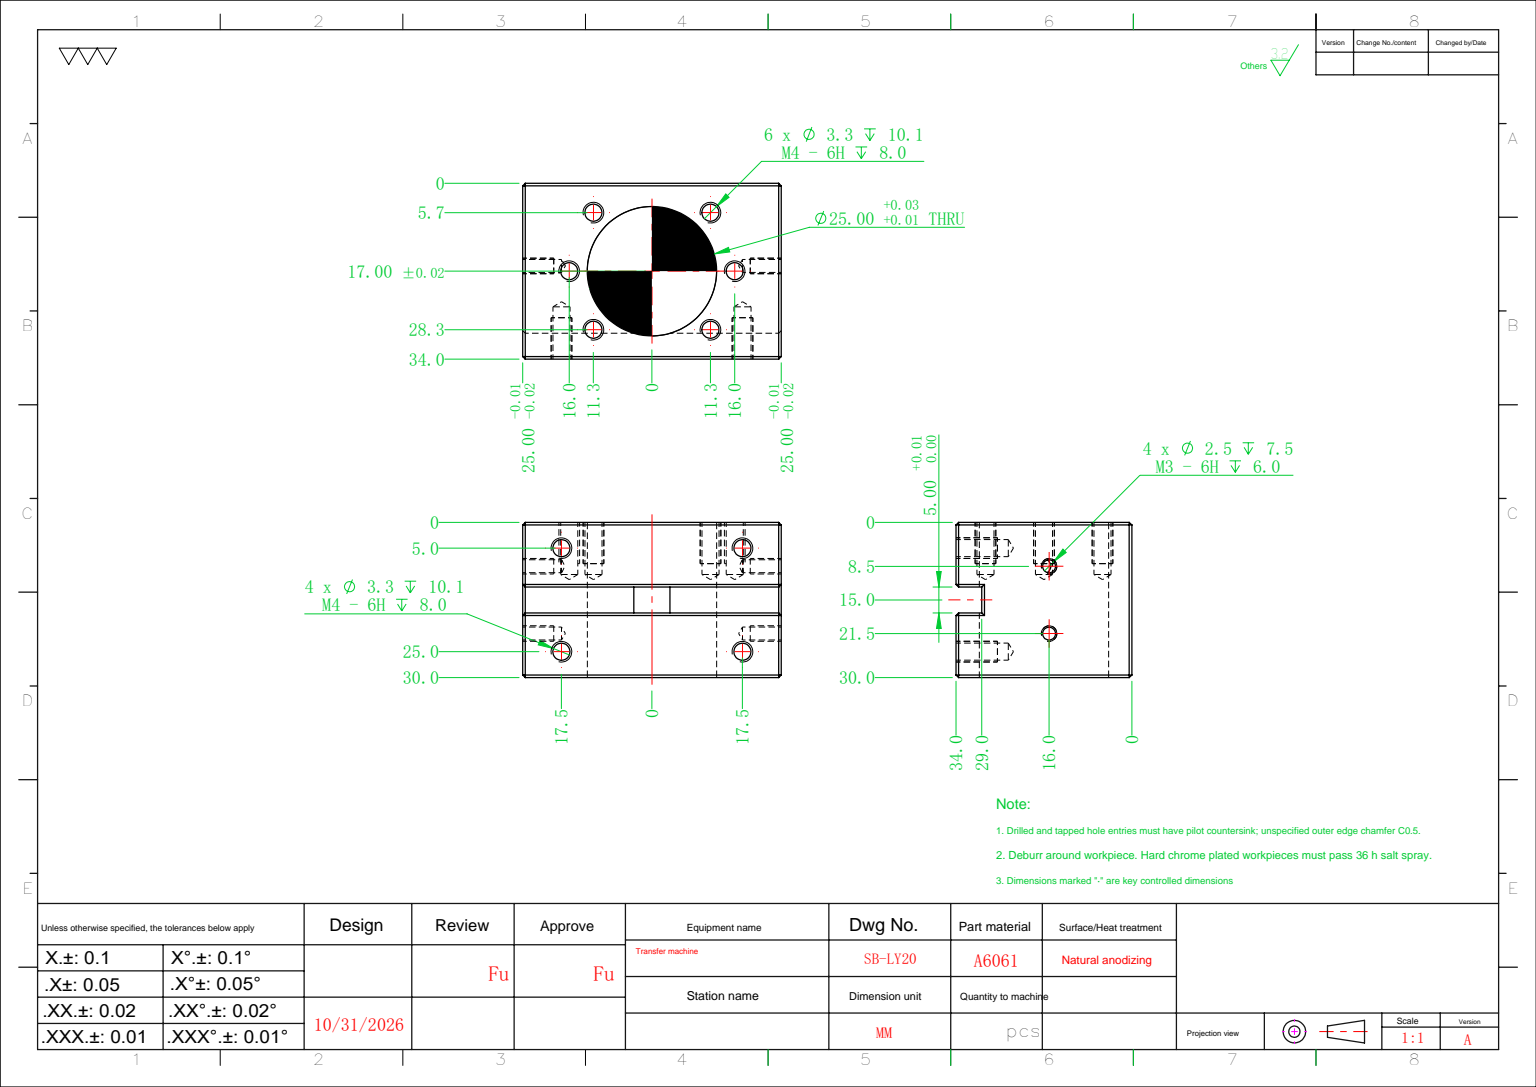
SolidWorks part; units mm, degrees
ref_plane "前视基准面" through (0, 0, 0) normal (0, 0, 1) x (1, 0, 0)
ref_plane "上视基准面" through (0, 0, 0) normal (0, 1, 0) x (1, 0, 0)
ref_plane "右视基准面" through (0, 0, 0) normal (1, 0, 0) x (0, 0, -1)
sketch "草图1" plane through (0, 0, 0) normal (0, 0, 1) x (1, 0, 0)
  line L1 (-25, -17) -> (25, -17)
  line L2 (-25, -17) -> (-25, 17)
  line L3 (-25, 17) -> (25, 17)
  line L4 (25, -17) -> (25, 17)
  line L5 (-25, -17) -> (25, 17) construction
  line L6 (-25, 17) -> (25, -17) construction
  point P0 (0, 0)
  dimension "D1" = 50
  dimension "D2" = 34
extrude "凸台-拉伸1" add sketch "草图1" along normal blind 30
hole_wizard "M4 螺纹孔1" positions "草图7" profile "草图8" tap size "M4" standard "ISO"
sketch "草图7" plane through (0, 0, 0) normal (0, 0, -1) x (-1, 0, 0)
  line L7 (0, 0) -> (0, 26.8833) construction
  line L9 (-16, 0) -> (16, 0) construction
  circle A0 centre (0, 0) radius 16 construction
  point P0 (-11.3137, -11.3137)
  point P3 (-16, 0)
  point P6 (-11.3137, 11.3137)
  point P9 (11.3137, 11.3137)
  point P12 (16, 0)
  point P15 (11.3137, -11.3137)
  dimension "D1" = 32
  dimension "D2" = 32
  dimension "D3" = 22.6274
sketch "草图8" plane through (11.3137, -11.3137, 0) normal (1, 0, 0) x (0, 1, 0)
  line L0 (0, 0) -> (0, 11.0914)
  line L1 (0, 11.0914) -> (1.65, 10.1)
  line L2 (1.65, 10.1) -> (1.65, 0)
  line L5 (1.65, 0) -> (0, 0)
  line L10 (0, 11.0914) -> (-1.65, 10.1) construction
  line L11 (0, -6.35) -> (0, 107.95) construction
  dimension "螺纹孔钻头直径" = 3.3
  dimension "螺纹孔钻头深度" = 10.1
  dimension "导头角度" = 118
cosmetic thread "孔螺蚊线1" parameters "D1"=8, "D2"=4
cosmetic thread "孔螺蚊线2" parameters "D1"=8, "D2"=4
cosmetic thread "孔螺蚊线3" parameters "D1"=8, "D2"=4
cosmetic thread "孔螺蚊线4" parameters "D1"=8, "D2"=4
cosmetic thread "孔螺蚊线5" parameters "D1"=8, "D2"=4
cosmetic thread "孔螺蚊线6" parameters "D1"=8, "D2"=4
hole_wizard "M3 螺纹孔1" positions "草图11" profile "草图12" tap size "M3" standard "ISO"
sketch "草图11" plane through (-25, 0, 0) normal (-1, 0, 0) x (0, 0, 1)
  line L8 (30, 17) -> (30, -17) construction
  line L9 (30, -17) -> (0, -17) construction
  point P0 (8.5, -1)
  point P2 (21.5, -1)
  dimension "D1" = 13
  dimension "D2" = 8.5
  dimension "D3" = 16
sketch "草图12" plane through (-25, -1, 8.5) normal (0, 1, 0) x (0, 0, 1)
  line L0 (0, 0) -> (0, 8.2511)
  line L1 (0, 8.2511) -> (1.25, 7.5)
  line L2 (1.25, 7.5) -> (1.25, 0)
  line L5 (1.25, 0) -> (0, 0)
  line L10 (0, 8.2511) -> (-1.25, 7.5) construction
  line L11 (0, -6.35) -> (0, 107.95) construction
  dimension "螺纹孔钻头直径" = 2.5
  dimension "螺纹孔钻头深度" = 7.5
  dimension "导头角度" = 118
cosmetic thread "孔螺蚊线9" parameters "D1"=6, "D2"=3
cosmetic thread "孔螺蚊线10" parameters "D1"=6, "D2"=3
mirror "镜向1" about plane through (0, 0, 0) normal (1, 0, 0) of "M3 螺纹孔1"
sketch "草图15" plane through (0, 0, 30) normal (0, 0, 1) x (1, 0, 0)
  line L0 (0, 0) -> (0, 32.7789) construction
  circle A0 centre (0, 0) radius 12.5
  dimension "D1" = 25
extrude "切除-拉伸1" cut sketch "草图15" against normal through all
hole_wizard "M4 螺纹孔2" positions "草图16" profile "草图17" tap size "M4" standard "ISO"
sketch "草图16" plane through (0, 17, 0) normal (0, 1, 0) x (1, 0, 0)
  line L0 (0, 0) -> (0, -30) construction
  line L1 (25, -30) -> (-25, -30) construction
  line L2 (25, -15) -> (-25, -15) construction
  line L3 (25, -30) -> (25, 0) construction
  line L4 (-25, -30) -> (-25, 0) construction
  point P0 (17.5, -25)
  point P3 (-17.5, -25)
  point P6 (-17.5, -5)
  point P9 (17.5, -5)
  dimension "D1" = 35
  dimension "D3" = 20
sketch "草图17" plane through (17.5, 17, 25) normal (1, 0, 0) x (0, 0, 1)
  line L0 (0, 0) -> (0, 11.0914)
  line L1 (0, 11.0914) -> (1.65, 10.1)
  line L2 (1.65, 10.1) -> (1.65, 0)
  line L5 (1.65, 0) -> (0, 0)
  line L10 (0, 11.0914) -> (-1.65, 10.1) construction
  line L11 (0, -6.35) -> (0, 107.95) construction
  dimension "螺纹孔钻头直径" = 3.3
  dimension "螺纹孔钻头深度" = 10.1
  dimension "导头角度" = 118
cosmetic thread "孔螺蚊线11" parameters "D1"=8, "D2"=4
cosmetic thread "孔螺蚊线12" parameters "D1"=8, "D2"=4
cosmetic thread "孔螺蚊线13" parameters "D1"=8, "D2"=4
cosmetic thread "孔螺蚊线14" parameters "D1"=8, "D2"=4
sketch "草图18" plane through (0, 17, 0) normal (0, 1, 0) x (1, 0, 0)
  line L0 (25, -30) -> (25, 0) construction
  line L1 (25, -17.5) -> (-25, -17.5)
  line L2 (25, -17.5) -> (25, -12.5)
  line L3 (25, -12.5) -> (-25, -12.5)
  line L4 (-25, -17.5) -> (-25, -12.5)
  line L5 (-25, -30) -> (-25, 0) construction
  line L6 (-25, -15) -> (25, -15) construction
  dimension "D1" = 5
extrude "切除-拉伸2" cut sketch "草图18" against normal blind 5
chamfer "倒角1" distance 0.5 angle 45 22 edges at (0, -17, 30) (0, -17, 0) (0, 17, 0) (0, 17, 12.5) (0, 17, 30) (-25, 0, 30) (-25, -17, 15) (-25, 0, 0) (-25, 17, 6.25) (-25, 14.5, 12.5) (-25, 12, 15) (-25, 14.5, 17.5) (-25, 17, 23.75) (0, 17, 17.5) (25, 14.5, 12.5) (25, 17, 6.25) (25, 0, 0) (25, -17, 15) (25, 0, 30) (25, 17, 23.75) (25, 14.5, 17.5) (25, 12, 15)
